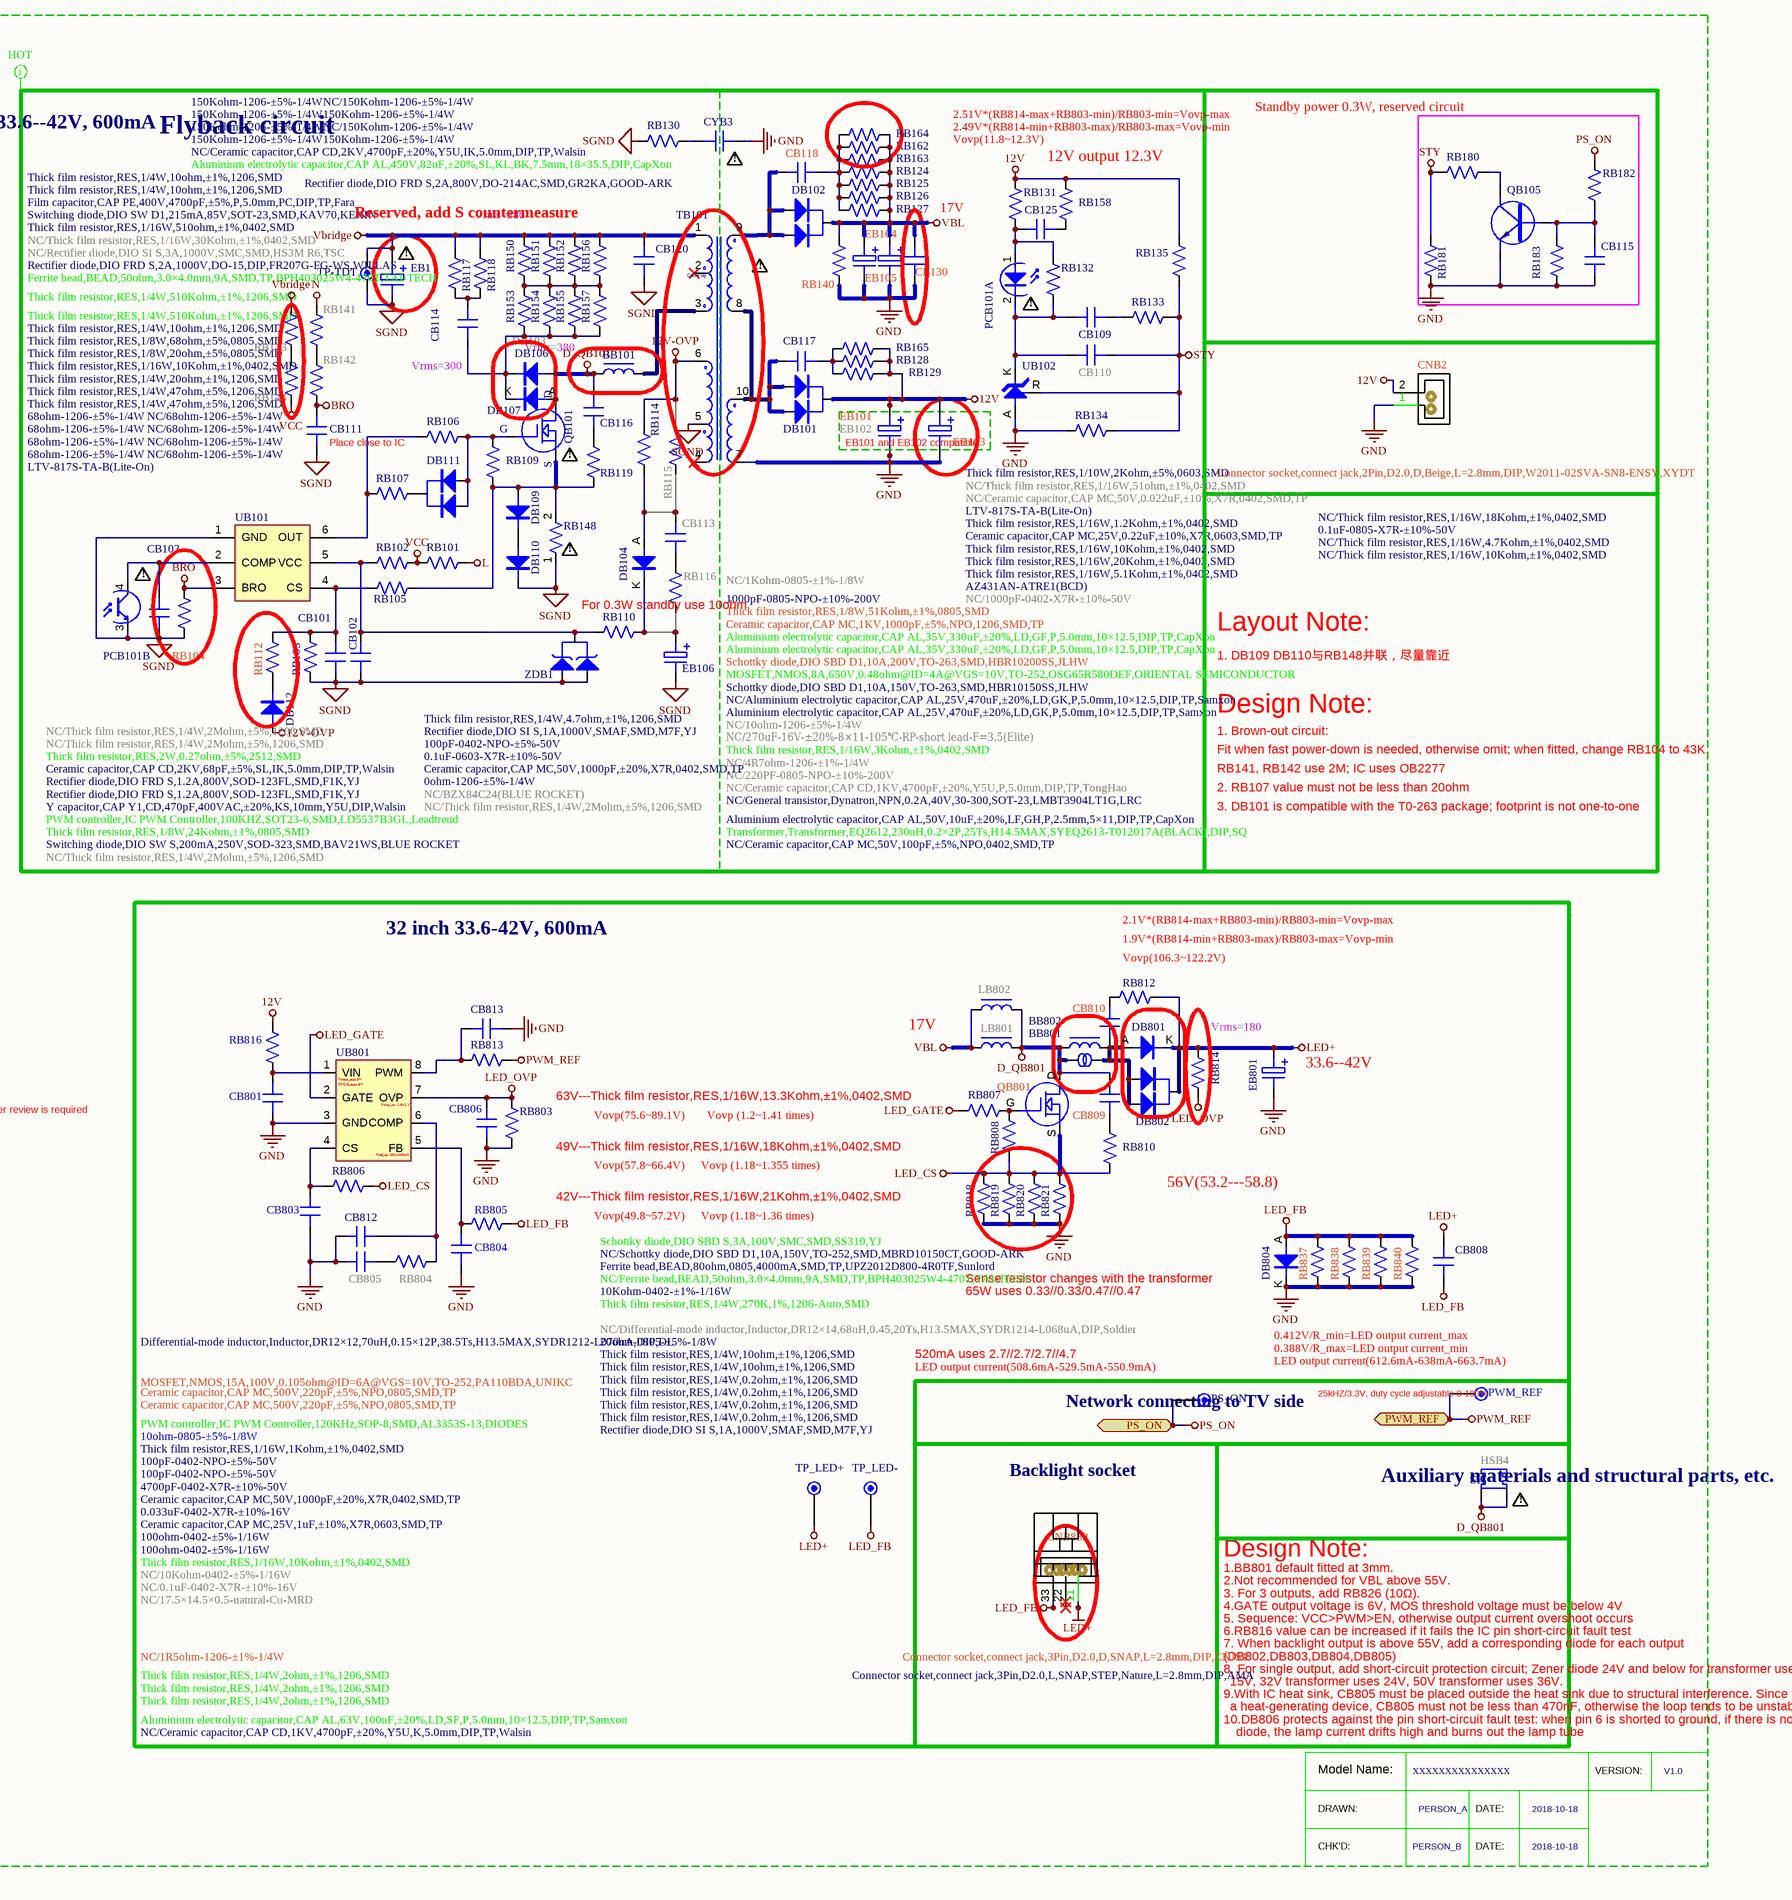
[diagram p0: MISC86383-5.SchDoc, right]
# Altium project MISC86383-33.PrjPCB (part 8 of 8)

## Sheet MISC86383-5.SchDoc: MISC86383 (continued)

### Library data of the parts
BB101 BB802 = 004.004.0001046-D: Ferrite bead,BEAD,50ohm,3.0×4.0,9A,SMD,TP,SMB-302540-K5B-L1,SOLDIER-D
BB801 = 004.004.0000346-D: Ferrite bead,BEAD,80ohm,0805,4000mA,SMD,TP,UPZ2012D800-4R0TF,Sunlord-D
CB101 CB111 CB803 CB813 = 100pF-0402-NPO-±5%-50V-D
CB102 CB109 = 0.1uF-0603-X7R-±10%-50V-D: CAP
CB103 = 1000pF-0402-X7R-±10%-50V-D
CB110 CB125 CB806 = 1000pF-0402-X7R-±10%-50V-D: CAP
CB113 = 220PF-0805-NPO-±10%-200V-D: CAP
CB114 = C242G472J20A201(编带/法拉)-DAI: CAP
CB115 = 0.1uF-0805-X7R-±10%-50V-D: CAP
CB116 = 004.003.0001889-DHAI: Ceramic capacitor,CAP CD,1KV,100pF,±5%,SL,OK,5.0mm,DIP,TP,TDK-DHAI
CB117 = 1000pF-0805-NPO-±10%-200V-D: CAP
CB118 = 陶瓷电容,CAP MC,1KV,4700pF,±10%,X7R,1206,SMD,TP,ISND-D
CB120 CB808 = 004.003.0001665: Ceramic capacitor,CAP CD,1KV,4700pF,±20%,Y5U,K,5.0mm,DIP,TP,Walsin-DHAI
CB130 = 004.003.0000886: Ceramic capacitor,CAP CD,1KV,4700pF,±20%,Y5U,P,5.0mm,DIP,TP,TongHao-DHAI
CB801 = 1uf-0603-X7R-±10%-25V-D
CB804 = 4700pF-0402-X7R-±10%-50V-D
CB805 = 0.1uF-0402-X7R-±10%-16V-D
CB809 CB810 = 004.003.0001392: Ceramic capacitor,CAP MC,500V,47pF,±5%,NPO,0805,SMD,TP,WALSIN-D
CB812 = 0.033uF-0402-X7R-±10%-16V-D
CNB1 = 连接插座,connect jack,2Pin,D8.6,L,SNAP,Fool-proofing,Black,L=4.0mm,DIP,YQ-DLMI: AC插座-八字侧出
CNB2 = XXX.XXX.0001753: Connector socket,connect jack,2Pin,D2.0,D,L=2.8mm,DIP,AMA-DHMI
CNB832 = XXX.XXX.0001754: Connector socket,connect jack,3Pin,D2.0,D,L=2.8mm,DIP,AMA-DHMI
CNB833 = XXX.XXX.0001725-DLMI: Connector socket,connect jack,3Pin,D2.0,L,SNAP,STEP,Nature,L=2.8mm,DIP,AMA-DLMI
Conformal_Coating = 三防漆,25kg/Can,Peters
CXB1 = X电容,CAP X2,MP,275VAC,0.47uF,±10%,S,15mm-Mini,PC,DIP,BM-DHMI: CAP
CYB1-CYB3 CYB6 = Y电容,CAP Y1,CD,470pF,400VAC,±20%,KS,10mm,Y5U,DIP,Walsin-DHMI: Y1 capacitor
DB1 = 004.005.0000860-D: Bridge rectifier,DIO BRD,3A,800V,YBS,SMD,YBS3010A,YJ-D
DB101 = 004.005.0000140-D: Rectifier diode,DIO SI D1,10A,150V,TO-263,SMD,MBRB10150CT,GOOD-ARK-D
DB102 = 004.005.0000473: Rectifier diode,DIO FRD D1,10A,400V,TO-263,SMD,MURB1040S,GOOD-ARK-D
DB103 = 整流二极管,DIO SI S,3A,1000V,SMC,SMD,HS3M R6,TSC-D: Diode
DB104 DB804 = M7(WEJ)-D: Diode
DB106 = RL207G(编带/GOOD-ARK)-DLAI: Diode
DB107 = 004.005.0000177-D: Rectifier diode,DIO SI S,1A,1000V,DO-214AC,SMD,M7,WEJ-D
DB109 DB110 = 整流二极管,DIO FRD S,1.2A,800V,eSGA,SMD,R12K,GOOD-ARK-D
DB111 = LBAV70LT1G(LRC)-D: Diode
DB112 = BAV21WS-D: Diode
DB801 = 004.005.0000432-D: Rectifier diode,DIO SI S,3A,1000V,SMC,SMD,GS3M,GULF-D
DB802 = 004.005.0000494-D: Schottky diode,DIO SBD D1,10A,150V,TO-252,SMD,MBRD10150CT,GOOD-ARK-D
EB1 = 004.003.0000164-DLMI: Aluminium electrolytic capacitor,CAP AL,400V,120uF,±20%,KM,BK,7.5mm,18×35.5,DIP,CapXon-DLMI
EB101 EB103 = 470uF-25V-±20%-10×12.5-105℃-GF-编带-F=5.0(CapXon)-DHAI: Electrolytic
EB102 = 270uF-16V-±20%-8×11-105℃-RP-短脚-F=3.5(Elite)-DHMI: CAP
EB104 EB105 = 100uF-63V-±20%-10×12.5-105℃-GF-编带-F=5.0(CapXon)-DHAI: Electrolytic
EB106 = 10uF-50V-±20%-5×11-105℃-GH-编带-F=2.5(CapXon)-DHAI: Electrolytic
EB801 = 47uF-100V-±20%-10×12-105℃-EV-编带-F=5.0(Elite)-DHAI: Electrolytic
FB1 = 004.026.0000010-DHMI: Slow-blow fuse,FUSE T,P,3.15A,250VAC,8.5×4.0×8mm,DIP,TP,Walter-DHMI
GL1 = 005.002.0000011: Silicone,0.2g,general,60,white,SLD-8854W,XY-DHMI
HSB1 HSB3-HSB5 = 17.5×14.5×0.5-本色-Cu-MRD-D: Heat sink
LB801 = SYDR1212-L003-EDL-DHMI: I-type inductor
LB802 = 差模电感,Inductor,DR12×14,68uH,0.45,20Ts,H13.5MAX,SYDR1214-L068uA,DIP,Soldier-DHMI: I-type inductor
LCB2 = 004.004.0002597-DHMI: Common-mode choke,Common Choke,UC1614,10.5mH±10%,0.15×1.0mm,48Ts,H14.0MAX,SYUC16-L10.5mA,DIP,CH-DHMI
MOVB1 = TVR10561KSW(为勤)-DHMI: Varistor
NTCB1 = SCK102R55AMBY502(短脚/为勤)-DHMI: Thermistor
PCB101 = LTV-817S-TA-B(光宝)-DMI: Optocoupler
PWM_REF TP-TDT TP_LED+ TP_LED- = TEST
QB101 = 004.007.0000227-D: MOSFET,NMOS,13.7A,650V,0.22ohm@ID=6.9A@VGS=10V,D2PAK,TK14G65W,TOSHIBA-D
QB105 = LMBT3904LT1G-D-NPN: Q-NPN-#-#-#
QB801 = AOD4454(AOS)-D: N Channel Single MOSFET
RB1-RB4 RB160 = 1M2ohm-1206-±5%-1/4W-D: RES
RB101 RB102 = 330Kohm-1206-±5%-1/4W-D: RES
RB103 = 6K8ohm-0402-±1%-1/16W-D
RB104 = 27Kohm-0402-±1%-1/16W-D
RB105 = 510ohm-0402-±1%-1/16W-D
RB106 = 68ohm-0805-±5%-1/8W-D
RB107 RB807 = 20ohm-0805-±5%-1/8W-D: RES
RB109 RB133 RB182 RB808 = 10Kohm-0402-±1%-1/16W-D
RB110 RB116-RB119 RB810 RB812 = 10ohm-1206-±5%-1/4W-D: RES
RB112 RB140 = 51Kohm-0805-±1%-1/8W-D: RES
RB114 RB115 = 4R7ohm-1206-±1%-1/4W-D: RES
RB124-RB127 RB162-RB165 = 68ohm-1206-±5%-1/4W-D: RES
RB128 RB129 = 47ohm-1206-±5%-1/4W-D: RES
RB130 = 20ohm-1206-±5%-1/4W-D
RB131 = 2Kohm-0603-±5%-1/10W-D
RB132 RB806 = 1Kohm-0402-±1%-1/16W-D
RB134 = 4K7ohm-0402-±1%-1/16W-D: RES
RB135 = 18Kohm-0402-±1%-1/16W-D: RES
RB141-RB144 = 2Mohm-1206-±5%-1/4W-D: RES
RB148 = 004.002.0001050: Thick film resistor,RES,2W,0.22ohm,±5%,2512,SMD-D
RB150-RB157 = 100Kohm-1206-±5%-1/4W-D: RES
RB158 = 3Kohm-0402-±1%-1/16W-D
RB180 = 20Kohm-0402-±1%-1/16W-D
RB181 = 1Kohm-0805-±1%-1/8W-D
RB183 = 4K7ohm-0402-±1%-1/16W-D
RB803 = 9K1ohm-0402-±1%-1/16W-D
RB804 = 10Kohm-0402-±5%-1/16W-D
RB805 = 100ohm-0402-±5%-1/16W-D: RES
RB813 = 100ohm-0402-±1%-1/16W-D
RB814 = 004.002.0001261: Thick film resistor,RES,1/4W,510Kohm,±1%,1206-Auto,SMD-D
RB816 = 33ohm-0805-±5%-1/8W-D
RB818-RB821 = 0R3ohm-1206-±5%-1/4W-D
RB837 RB838 = 1R5ohm-1206-±1%-1/4W-D: RES
RB839 = 2R2ohm-1206-±1%-1/4W-D: RES
RB840 = 1R6ohm-1206-±1%-1/4W-D: RES
TB101 = 004.004.0002512-DLMI: Transformer,Transformer,EQ2612,230uH,0.2×2P,25Ts,H14.5MAX,SYEQ2613Z-T012033A(BLACK),DIP,SQ-DLMI
UB101 = LD7537RGL(通嘉)-D: IC
UB102 = AZ431AN-ATRE1(BCD)-D: SMD 431
UB801 = OB3350CPA(OB)-D: IC
ZDB1 = LBZX84C24LT1G(LRC)-D: Diode

## Nets that join several sheets
1.15V_STB: MISC86383-11 (8 pins), MISC86383-12 (13 pins)
3V3_STB: MISC86383-11 (7 pins), MISC86383-12 (23 pins), MISC86383-18 (RK4.2 RK18.2)
3V3_TUNER: MISC86383-11 (7 pins), MISC86383-16 (LT12.1)
5V_M: MISC86383-11 (8 pins), MISC86383-13 (7 pins), MISC86383-19 (CL16.1 RL50.1 UL3.1)
5V_STB: MISC86383-11 (22 pins), MISC86383-12 (RV12.2 RV13.2), MISC86383-18 (RK1.2 RK13.1 RK15.1)
12V: MISC86383-11 (7 pins), MISC86383-15 (12 pins), MISC86383-19 (CM11.2 QM7.S), MISC86383-5 (14 pins)
GND: MISC86383-11 (52 pins), MISC86383-12 (54 pins), MISC86383-13 (61 pins), MISC86383-14 (18 pins), MISC86383-15 (25 pins), MISC86383-16 (46 pins), MISC86383-18 (13 pins), MISC86383-19 (74 pins), MISC86383-5 (35 pins)
PS_ON: MISC86383-11 (CG4.1 RG3.2 RG3.3), MISC86383-5 (PS_ON.1 RB182.2)
PWM_REF: MISC86383-11 (CG2.1 RG2.2 RG2.3), MISC86383-5 (PWM_REF.1 RB813.2)
VCC_DDR: MISC86383-11 (6 pins), MISC86383-12 (7 pins)
VCC_PANEL: MISC86383-11 (5 pins), MISC86383-19 (5 pins)
AC_OFF_DET: MISC86383-11 (QA3.C), MISC86383-12 (RR6.2)
AMP-LO: MISC86383-12 (U1.46), MISC86383-15 (RA21.1)
AMP-MUTE: MISC86383-12 (U1.59), MISC86383-15 (RA1.2 RA8.1)
AMP-RO: MISC86383-12 (U1.47), MISC86383-15 (RA5.1)
AV1_LIN: MISC86383-12 (U1.37), MISC86383-13 (CI9.1)
AV1_RIN: MISC86383-12 (U1.36), MISC86383-13 (CI6.1)
AV2_LIN: MISC86383-12 (U1.41), MISC86383-13 (CI4.1)
AV2_RIN: MISC86383-12 (U1.40), MISC86383-13 (CI3.1)
CPV/: MISC86383-12 (CF4.1 U1.104), MISC86383-19 (RG25.1 RG59.1)
CVBS_IN: MISC86383-12 (U1.32), MISC86383-13 (CI8.1)
CVBS_IN/OUT: MISC86383-12 (RI39.1), MISC86383-13 (5 pins)
CVBS_OUT: MISC86383-12 (U1.34), MISC86383-13 (CO9.2 RO12.1 RO14.2)
DDC_SCL/UART_RX: MISC86383-12 (6 pins), MISC86383-13 (DV3.K RV22.1), MISC86383-14 (RH2.2)
DDC_SDA/UART_TX: MISC86383-12 (6 pins), MISC86383-13 (DV4.K RV23.1), MISC86383-14 (RH1.2)
EXE_IR: MISC86383-12 (U1.63), MISC86383-13 (RO6.2 RO9.2 RO10.2)
GIN0M: MISC86383-12 (U1.23), MISC86383-13 (CF33.1)
GVOFF/: MISC86383-12 (U1.106), MISC86383-19 (RG40.1 RGV1.1)
HD1_Y: MISC86383-12 (U1.28), MISC86383-13 (CI1.1)
HDMI2_DET: MISC86383-12 (U1.65), MISC86383-14 (RH28.1 RH29.1)
HDMI2_RX0_N: MISC86383-12 (U1.5), MISC86383-14 (AVH1.9)
HDMI2_RX0_P: MISC86383-12 (U1.6), MISC86383-14 (AVH1.7)
HDMI2_RX1_N: MISC86383-12 (U1.7), MISC86383-14 (AVH1.6)
HDMI2_RX1_P: MISC86383-12 (U1.8), MISC86383-14 (AVH1.4)
HDMI2_RX2_N: MISC86383-12 (U1.9), MISC86383-14 (AVH1.3)
HDMI2_RX2_P: MISC86383-12 (U1.10), MISC86383-14 (AVH1.1)
HDMI2_RXC_N: MISC86383-12 (U1.3), MISC86383-14 (AVH1.12)
HDMI2_RXC_P: MISC86383-12 (U1.4), MISC86383-14 (AVH1.10)
HDMI2_SCL: MISC86383-12 (U1.140), MISC86383-14 (RH10.1)
HDMI2_SDA: MISC86383-12 (U1.139), MISC86383-14 (RH11.1)
HDMI-CEC: MISC86383-12 (U1.143), MISC86383-14 (RH13.2)
HDMI_ARC: MISC86383-12 (U1.149), MISC86383-14 (CH15.2)
HOTPLUG2': MISC86383-12 (U1.145), MISC86383-14 (RPH2.6 RPH2.8)
IF_AGC: MISC86383-12 (U1.48), MISC86383-16 (CT19.2 RT2.2 RT18.2)
KEY: MISC86383-12 (U1.133), MISC86383-18 (CK2.1 RK3.1)
LED_RED: MISC86383-12 (U1.129), MISC86383-18 (RK18.1 RK20.2 RK21.1)
LINE_L_OUT: MISC86383-12 (U1.44), MISC86383-13 (RO1.1)
LINE_R_OUT: MISC86383-12 (U1.45), MISC86383-13 (RO5.1)
M_SCL_IC: MISC86383-12 (RF6.1 U1.57), MISC86383-16 (DT3.K RT6.2), MISC86383-19 (RG60.1)
M_SDA_IC: MISC86383-12 (RF7.1 U1.56), MISC86383-16 (DT2.K RT5.2), MISC86383-19 (RG61.1)
mLV0N: MISC86383-12 (U1.99), MISC86383-19 (CN1.3)
mLV0P: MISC86383-12 (U1.100), MISC86383-19 (CN1.2)
mLV1N: MISC86383-12 (U1.97), MISC86383-19 (CN1.5)
mLV1P: MISC86383-12 (U1.98), MISC86383-19 (CN1.4)
mLV2N: MISC86383-12 (U1.95), MISC86383-19 (CN1.7)
mLV2P: MISC86383-12 (U1.96), MISC86383-19 (CN1.6)
mLV3N: MISC86383-12 (U1.90), MISC86383-19 (CN1.13)
mLV3P: MISC86383-12 (U1.91), MISC86383-19 (CN1.12)
mLV4N: MISC86383-12 (U1.88), MISC86383-19 (CN1.15)
mLV4P: MISC86383-12 (U1.89), MISC86383-19 (CN1.14)
mLV5N: MISC86383-12 (U1.86), MISC86383-19 (CN1.17)
mLV5P: MISC86383-12 (U1.87), MISC86383-19 (CN1.16)
mLVCLKN: MISC86383-12 (U1.93), MISC86383-19 (CN1.10)
mLVCLKP: MISC86383-12 (U1.94), MISC86383-19 (CN1.9)
OE1/: MISC86383-12 (CF11.1 U1.105), MISC86383-19 (RG46.1)
Panel_DVDD_EN_IC: MISC86383-12 (U1.64), MISC86383-19 (RL7.2 RL51.1)
PANEL_ON: MISC86383-11 (DM1.A QM6.C RM5.1 RM7.1), MISC86383-19 (DM3.A RM12.1)
PANEL_ON/OFF: MISC86383-11 (RM8.1 RM10.1), MISC86383-12 (U1.60)
POL/: MISC86383-12 (CF12.1 U1.108), MISC86383-19 (RG52.1)
POW_EN: MISC86383-11 (RM3.2 RM4.2), MISC86383-12 (U1.120)
PWM0: MISC86383-11 (RG2.1), MISC86383-12 (RF13.1 RF14.2 U1.109)
PWM1: MISC86383-11 (RG3.1), MISC86383-12 (RF18.1 U1.110)
REMOTE: MISC86383-12 (U1.111), MISC86383-18 (CK6.2 RK16.1)
STV/: MISC86383-12 (CF3.1 U1.107), MISC86383-19 (RG26.1)
TCON6: MISC86383-12 (CF8.1 U1.102), MISC86383-19 (RG62.1)
TP/: MISC86383-12 (CF6.1 U1.103), MISC86383-19 (RG78.1)
USB0_DM/: MISC86383-12 (U1.70), MISC86383-13 (CU5.2 CU5.3 DU2.K)
USB0_DP/: MISC86383-12 (U1.71), MISC86383-13 (CU6.2 CU6.3 DU1.K)
VGA_BIN: MISC86383-12 (U1.21), MISC86383-13 (CV7.1)
VGA_GIN: MISC86383-12 (U1.22), MISC86383-13 (CV3.1)
VGA_HS: MISC86383-12 (U1.20), MISC86383-13 (CV9.2 RV6.2)
VGA_RIN: MISC86383-12 (U1.24), MISC86383-13 (CV1.1)
VGA_VS: MISC86383-12 (U1.25), MISC86383-13 (CV10.2 RV10.2)
VIFM: MISC86383-12 (U1.50), MISC86383-16 (CT23.2)
VIFP: MISC86383-12 (U1.49), MISC86383-16 (CT20.2)
XTAL_O: MISC86383-12 (LF1.2), MISC86383-16 (CT14.2 UT1.13 YT1.1)